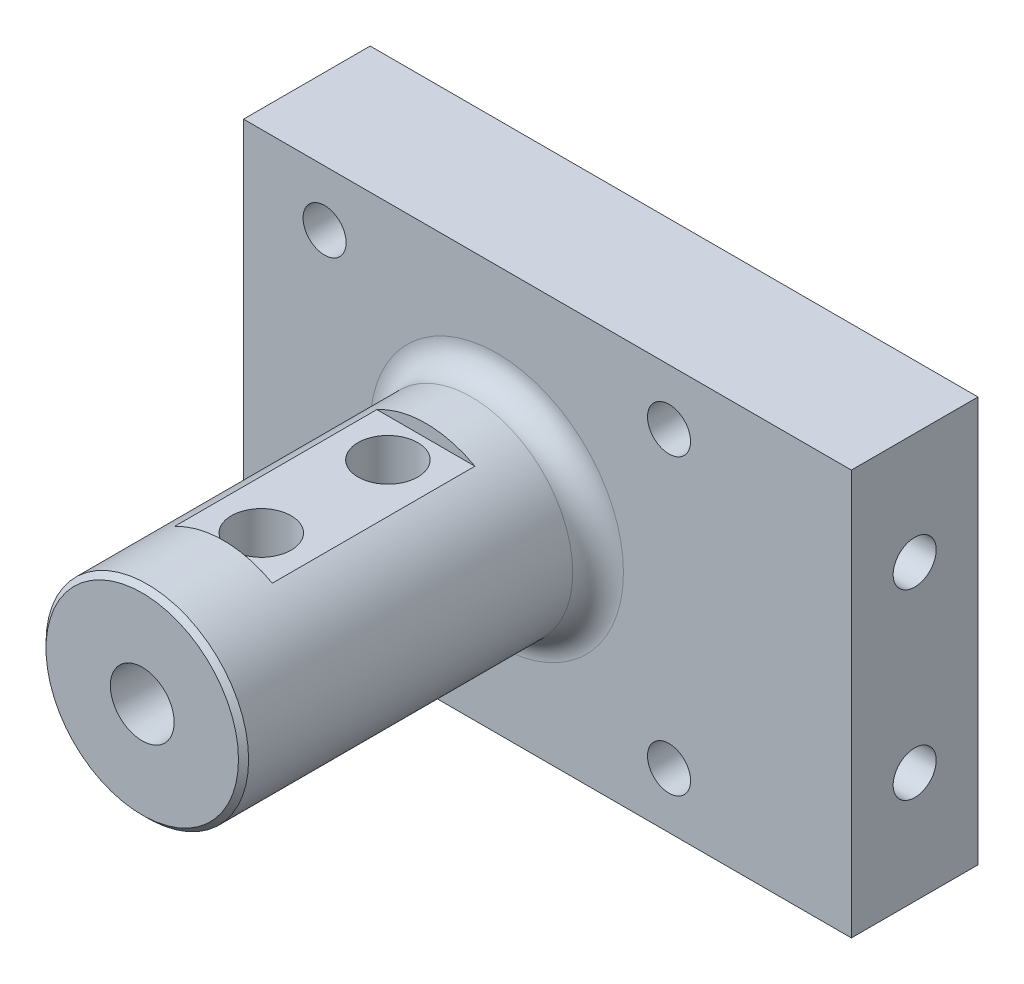
SolidWorks part; units mm, degrees
material "T2"
ref_plane "前视基准面" through (0, 0, 0) normal (0, 0, 1) x (1, 0, 0)
ref_plane "上视基准面" through (0, 0, 0) normal (0, 1, 0) x (1, 0, 0)
ref_plane "右视基准面" through (0, 0, 0) normal (1, 0, 0) x (0, 0, -1)
sketch "草图13" plane through (0, 0, 0) normal (0, 0, 1) x (1, 0, 0)
  line L1 (-50, -40) -> (50, -40)
  line L2 (-50, -40) -> (-50, 40)
  line L3 (-50, 40) -> (50, 40)
  line L4 (50, -40) -> (50, 40)
  line L5 (0, 40) -> (0, -40) construction
  line L6 (-50, 0) -> (50, 0) construction
  point P0 (0, 0)
  dimension "D1" = 100
  dimension "D2" = 80
extrude "凸台-拉伸3" add sketch "草图13" along normal blind 25
sketch "草图14" plane through (0, 0, 25) normal (0, 0, 1) x (1, 0, 0)
  line L1 (-34, -29) -> (34, -29) construction
  line L2 (-34, -29) -> (-34, 29) construction
  line L3 (-34, 29) -> (34, 29) construction
  line L4 (34, -29) -> (34, 29) construction
  line L5 (0, 29) -> (0, -29) construction
  line L6 (-34, 0) -> (34, 0) construction
  circle A0 centre (-34, 29) radius 0.5
  circle A1 centre (34, 29) radius 0.5
  circle A2 centre (34, -29) radius 0.5
  circle A3 centre (-34, -29) radius 0.5
  point P0 (0, 0)
  dimension "D3" = 1
  dimension "D1" = 68
  dimension "D2" = 58
extrude "切除-拉伸4" cut sketch "草图14" against normal blind 18
sketch "草图15" plane through (0, 0, 25) normal (0, 0, 1) x (1, 0, 0)
  circle A0 centre (0, 0) radius 20
  dimension "D1" = 40
extrude "凸台-拉伸4" add sketch "草图15" along normal blind 70
hole_wizard "Ø10.0 (10) 直径孔1" positions "草图16" profile "草图17" hole size "Ø10.0" standard "GB"
sketch "草图16" plane through (0, 0, 95) normal (0, 0, 1) x (1, 0, 0)
  point P5 (0, 0)
sketch "草图17" plane through (0, 0, 95) normal (1, 0, 0) x (0, -1, 0)
  line L0 (0, 0) -> (0, 28.0043)
  line L1 (0, 28.0043) -> (5, 25)
  line L2 (5, 25) -> (5, 0)
  line L5 (5, 0) -> (0, 0)
  line L10 (0, 28.0043) -> (-5, 25) construction
  line L11 (0, -6.35) -> (0, 107.95) construction
  dimension "孔直径" = 10
  dimension "孔深度" = 25
  dimension "导头角度" = 118
sketch "草图19" plane through (0, 0, 0) normal (0, 1, 0) x (1, 0, 0)
  line L0 (0, -95) -> (0, 0) construction
  line L1 (-20, -95) -> (20, -95) construction
  line L2 (0, -95) -> (-0.5, -95) construction
  line L3 (-0.5, -95) -> (0, -85) construction
  line L4 (0, -95) -> (-0.5, -95)
  line L5 (-6.3, -95) -> (-5.65, -82)
  line L6 (-5.65, -82) -> (-5, -82)
  line L8 (-5, -82) -> (-5, -95)
  line L10 (0, -95) -> (-0.5, -95)
  line L11 (-5, -70) -> (-5, -95) construction
  line L12 (-5, -95) -> (-6.3, -95)
  dimension "D1" = 0.5
  dimension "D2" = 10
  dimension "D3" = 12.6
  dimension "D4" = 13
revolve "切除-旋转10" cut sketch "草图19" angle 360 about L0
ref_plane "基准面3" through (0, 0, 79) normal (0, 0, 1) x (1, 0, 0)
sketch "草图21" plane through (0, 0, 79) normal (0, 0, 1) x (1, 0, 0)
  line L1 (-27.2886, -17.5) -> (27.2886, -17.5)
  line L2 (-27.2886, -17.5) -> (-27.2886, 17.5)
  line L3 (-27.2886, 17.5) -> (27.2886, 17.5)
  line L4 (27.2886, -17.5) -> (27.2886, 17.5)
  line L5 (0, 17.5) -> (0, -17.5) construction
  line L6 (-27.2886, 0) -> (27.2886, 0) construction
  point P0 (0, 0)
  dimension "D1" = 35
extrude "切除-拉伸5" cut sketch "草图21" against normal blind 40 flip side to cut
hole_wizard "G1/4 螺纹孔1" positions "草图22" profile "草图23" tap size "G1/4" standard "GB"
sketch "草图22" plane through (0, 17.5, 0) normal (0, 1, 0) x (1, 0, 0)
  line L0 (0, 0) -> (0, -95) construction
  line L1 (-20, -95) -> (20, -95) construction
  line L2 (-9.6825, -59) -> (9.6825, -59) construction
  line L3 (-9.6825, -39) -> (-9.6825, -79) construction
  line L4 (9.6825, -79) -> (9.6825, -39) construction
  point P13 (0, -46.5)
  point P15 (0, -71.5)
  dimension "D1" = 25
sketch "草图23" plane through (0, 17.5, 71.5) normal (1, 0, 0) x (0, 0, 1)
  line L0 (0, 0) -> (0, 28.5451)
  line L1 (0, 28.5451) -> (5.9, 25)
  line L2 (5.9, 25) -> (5.9, 0)
  line L5 (5.9, 0) -> (0, 0)
  line L10 (0, 28.5451) -> (-5.9, 25) construction
  line L11 (0, -6.35) -> (0, 107.95) construction
  dimension "螺纹孔钻头直径" = 11.8
  dimension "螺纹孔钻头深度" = 25
  dimension "导头角度" = 118
cosmetic thread "孔螺蚊线5" parameters "D1"=20, "D2"=13.157
cosmetic thread "孔螺蚊线6" parameters "D1"=20, "D2"=13.157
chamfer "倒角1" distance 1 angle 45 1 edges at (20, 0, 95)
hole_wizard "M10 螺纹孔1" positions "草图24" profile "草图25" tap size "M10" standard "GB"
sketch "草图24" plane through (0, 0, 25) normal (0, 0, 1) x (1, 0, 0)
  point P4 (-34, 29)
  point P7 (34, 29)
  point P10 (34, -29)
  point P13 (-34, -29)
sketch "草图25" plane through (-34, 29, 25) normal (1, 0, 0) x (0, -1, 0)
  line L0 (0, 0) -> (0, 30.0537)
  line L1 (0, 30.0537) -> (4.25, 27.5)
  line L2 (4.25, 27.5) -> (4.25, 0)
  line L5 (4.25, 0) -> (0, 0)
  line L10 (0, 30.0537) -> (-4.25, 27.5) construction
  line L11 (0, -6.35) -> (0, 107.95) construction
  dimension "螺纹孔钻头直径" = 8.5
  dimension "螺纹孔钻头深度" = 27.5
  dimension "导头角度" = 118
cosmetic thread "孔螺蚊线7" parameters "D1"=18, "D2"=10
cosmetic thread "孔螺蚊线8" parameters "D1"=18, "D2"=10
cosmetic thread "孔螺蚊线9" parameters "D1"=18, "D2"=10
cosmetic thread "孔螺蚊线10" parameters "D1"=18, "D2"=10
fillet "圆角1" radius 5 1 edges at (-20, 0, 25)
ref_plane "基准面4" through (0, 0, 69) normal (0, 0, 1) x (1, 0, 0)
hole_wizard "M6 螺纹孔1" positions "草图26" profile "草图27" tap size "M6" standard "GB"
sketch "草图26" plane through (0, 0, 69) normal (0, 0, 1) x (1, 0, 0)
  point P0 (0, 0)
sketch "草图27" plane through (0, 0, 69) normal (1, 0, 0) x (0, -1, 0)
  line L0 (0, 0) -> (0, 36.5022)
  line L1 (0, 36.5022) -> (2.5, 35)
  line L2 (2.5, 35) -> (2.5, 0)
  line L5 (2.5, 0) -> (0, 0)
  line L10 (0, 36.5022) -> (-2.5, 35) construction
  line L11 (0, -6.35) -> (0, 107.95) construction
  dimension "螺纹孔钻头直径" = 5
  dimension "螺纹孔钻头深度" = 35
  dimension "导头角度" = 118
cosmetic thread "孔螺蚊线11" parameters "D1"=30, "D2"=6
sketch "草图35" plane through (50, 0, 0) normal (1, 0, 0) x (0, 0, -1)
  line L4 (0, -40) -> (0, 40)
  line L5 (0, 40) -> (-25, 40)
  line L6 (-25, 40) -> (-25, -40)
  line L7 (-25, -40) -> (0, -40)
  line L8 (0, -40) -> (0, 40)
  line L9 (0, 40) -> (-25, 40)
  line L10 (-25, 40) -> (-25, -40)
  line L11 (-25, -40) -> (0, -40)
  dimension "D1" = 0
extrude "凸台-拉伸7" add sketch "草图35" along normal blind 20
hole_wizard "M10 螺纹孔4" positions "草图36" profile "草图37" tap size "M10" standard "GB"
sketch "草图36" plane through (70, 0, 0) normal (1, 0, 0) x (0, 0, -1)
  line L0 (-12.5, -40) -> (-12.5, 40) construction
  line L1 (-25, -40) -> (0, -40) construction
  line L2 (-25, 0) -> (0, 0) construction
  line L3 (-25, 40) -> (-25, -40) construction
  point P16 (-12.5, -18)
  point P18 (-12.5, 18)
  point P21 (0, 0)
  point P22 (0, 0)
  dimension "D1" = 36
sketch "草图37" plane through (70, 18, 12.5) normal (0, 1, 0) x (0, 0, -1)
  line L0 (0, 0) -> (0, 30.0537)
  line L1 (0, 30.0537) -> (4.25, 27.5)
  line L2 (4.25, 27.5) -> (4.25, 0)
  line L5 (4.25, 0) -> (0, 0)
  line L10 (0, 30.0537) -> (-4.25, 27.5) construction
  line L11 (0, -6.35) -> (0, 107.95) construction
  dimension "螺纹孔钻头直径" = 8.5
  dimension "螺纹孔钻头深度" = 27.5
  dimension "导头角度" = 118
cosmetic thread "孔螺蚊线14" parameters "D1"=20, "D2"=10
cosmetic thread "孔螺蚊线15" parameters "D1"=20, "D2"=10
